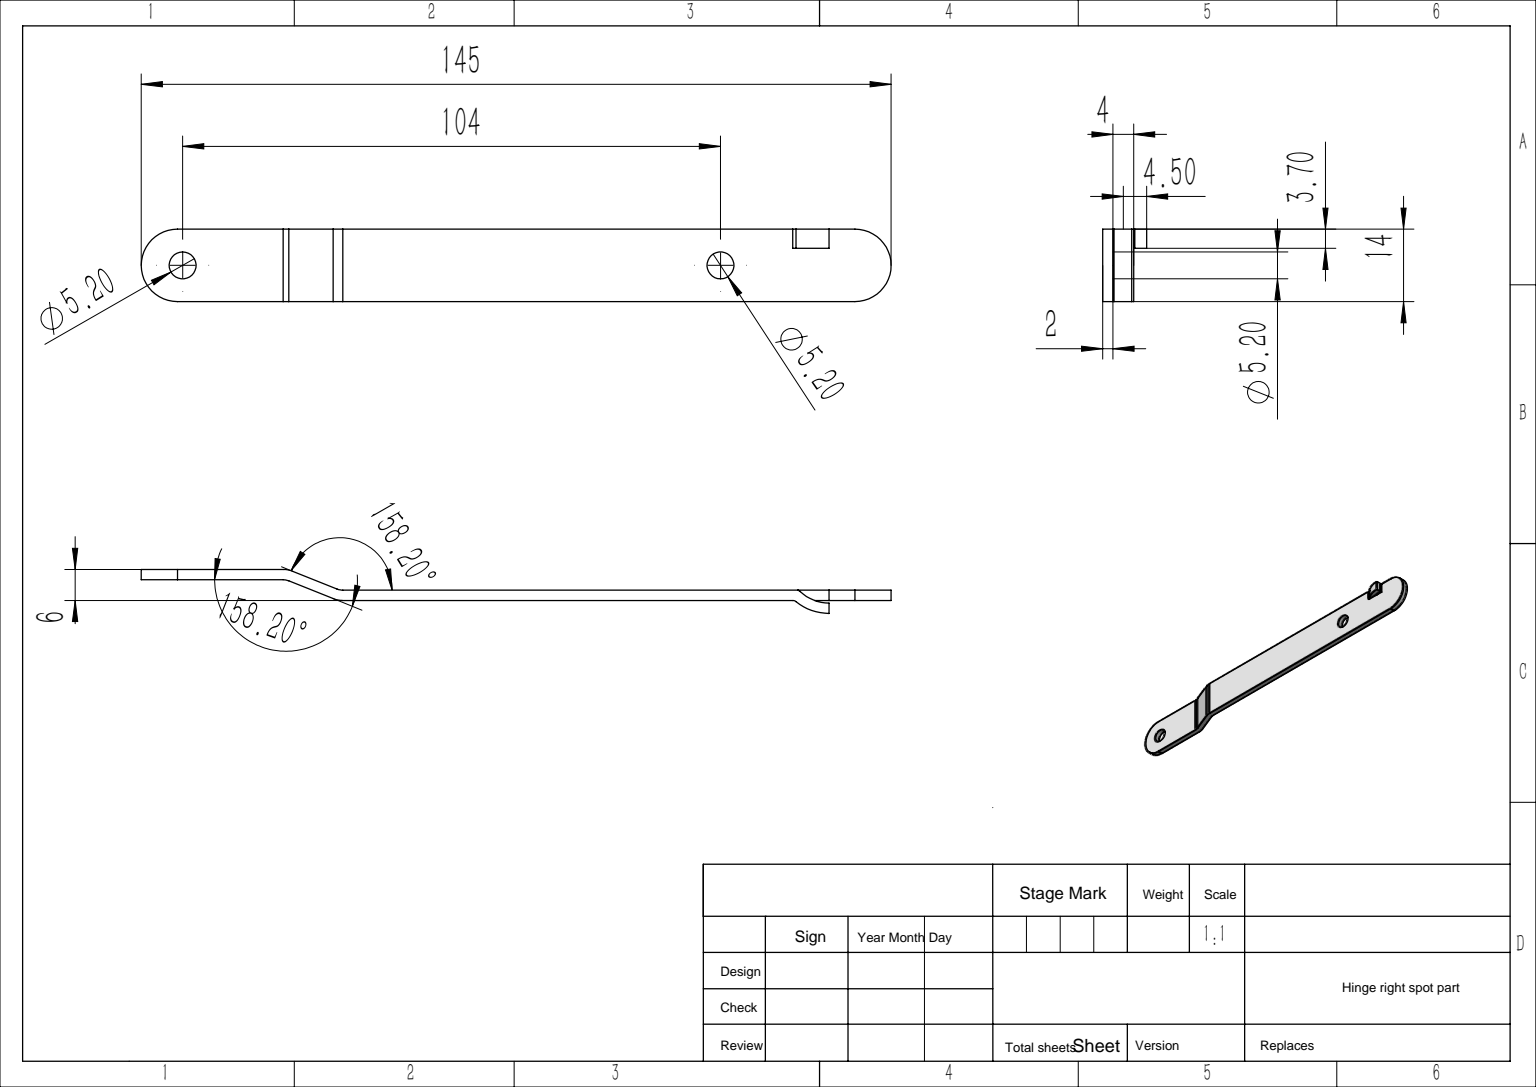
from build123d import *

# Parameters (mm, degrees)
EXTRUDE1_DEPTH      = 7
EXTRUDE2_DEPTH      = 146.223964964
EXTRUDE2_DEPTH_BACK = 146.223964964
SKETCH2_R           = 2.6
SKETCH5_W           = 6
SKETCH5_H           = 3.7
EXTRUDE5_DEPTH      = 146.292807805
EXTRUDE6_DEPTH      = 3.7


with BuildPart() as part:
    # Sketch1 → Extrude1 (new, symmetric)
    with BuildSketch(Plane.XY):
        with BuildLine():
            Line((0, 0), (27.422252789, 0))
            ThreePointArc((27.422252789, 0), (27.989575353, 0.05413084), (28.536424818, 0.214569927))
            Line((28.536424818, 0.214569927), (37.105958636, 3.642383454))
            ThreePointArc((37.105958636, 3.642383454), (38.017374412, 3.909781934), (38.962912018, 4))
            Line((38.962912018, 4), (145, 4))
            Line((145, 4), (145, 2))
            Line((145, 2), (38.962912018, 2))
            ThreePointArc((38.962912018, 2), (38.395589454, 1.94586916), (37.848739989, 1.785430073))
            Line((37.848739989, 1.785430073), (29.279206171, -1.642383454))
            ThreePointArc((29.279206171, -1.642383454), (28.367790395, -1.909781934), (27.422252789, -2))
            Line((27.422252789, -2), (0, -2))
            Line((0, -2), (0, 0))
        make_face()
    extrude(amount=EXTRUDE1_DEPTH, both=True)

    # Sketch2 → Extrude2 (cut, two sides: drawn at the far end of the back side and taken through both)
    with BuildSketch(Plane(origin=(0, 0, 0), x_dir=(1, 0, 0), z_dir=(0, 1, 0)).offset(-EXTRUDE2_DEPTH_BACK)):
        with Locations(Location((8, 0, 0), (0, 0, 270))):
            Circle(SKETCH2_R)
        with Locations(Location((112, 0, 0), (0, 0, 270))):
            Circle(SKETCH2_R)
        with BuildLine():
            Line((138, 7), (138, 13.502314884))
            Line((138, 13.502314884), (156.33198023, 13.502314884))
            Line((156.33198023, 13.502314884), (156.33198023, -14.26269046))
            Line((156.33198023, -14.26269046), (138, -14.26269046))
            Line((138, -14.26269046), (138, -7))
            ThreePointArc((138, -7), (145, 0), (138, 7))
        make_face()
        with BuildLine():
            Line((7, 7), (7, 12.663603668))
            Line((7, 12.663603668), (-7.097085647, 12.663603668))
            Line((-7.097085647, 12.663603668), (-7.097085647, -11.053510543))
            Line((-7.097085647, -11.053510543), (7, -11.053510543))
            Line((7, -11.053510543), (7, -7))
            ThreePointArc((7, -7), (0, 0), (7, 7))
        make_face()
    extrude(amount=EXTRUDE2_DEPTH + EXTRUDE2_DEPTH_BACK, mode=Mode.SUBTRACT)

    # Sketch5 → Extrude5 (cut, through all)
    with BuildSketch(Plane(origin=(0, 4, 0), x_dir=(1, 0, 0), z_dir=(0, 1, 0))):
        with Locations((130, 5.15)):
            Rectangle(SKETCH5_W, SKETCH5_H)
    extrude(amount=-EXTRUDE5_DEPTH, mode=Mode.SUBTRACT)

    # Sketch6 → Extrude6 (add)
    with BuildSketch(Plane.XY.offset(-7)):
        with BuildLine():
            Line((125.978380641, 4), (124.313573726, 4))
            Line((124.313573726, 4), (124.313573726, 2))
            Line((124.313573726, 2), (126.730778484, 2))
            ThreePointArc((126.730778484, 2), (127.10118691, 2.071131011), (127.418900283, 2.274404804))
            ThreePointArc((127.418900283, 2.274404804), (129.995755169, 3.923082851), (133, 4.5))
            Line((133, 4.5), (133, 6.5))
            ThreePointArc((133, 6.5), (129.608718605, 5.914287154), (126.61035388, 4.22500979))
            ThreePointArc((126.61035388, 4.22500979), (126.313798135, 4.057930414), (125.978380641, 4))
        make_face()
    extrude(amount=EXTRUDE6_DEPTH)


solid = part.part
